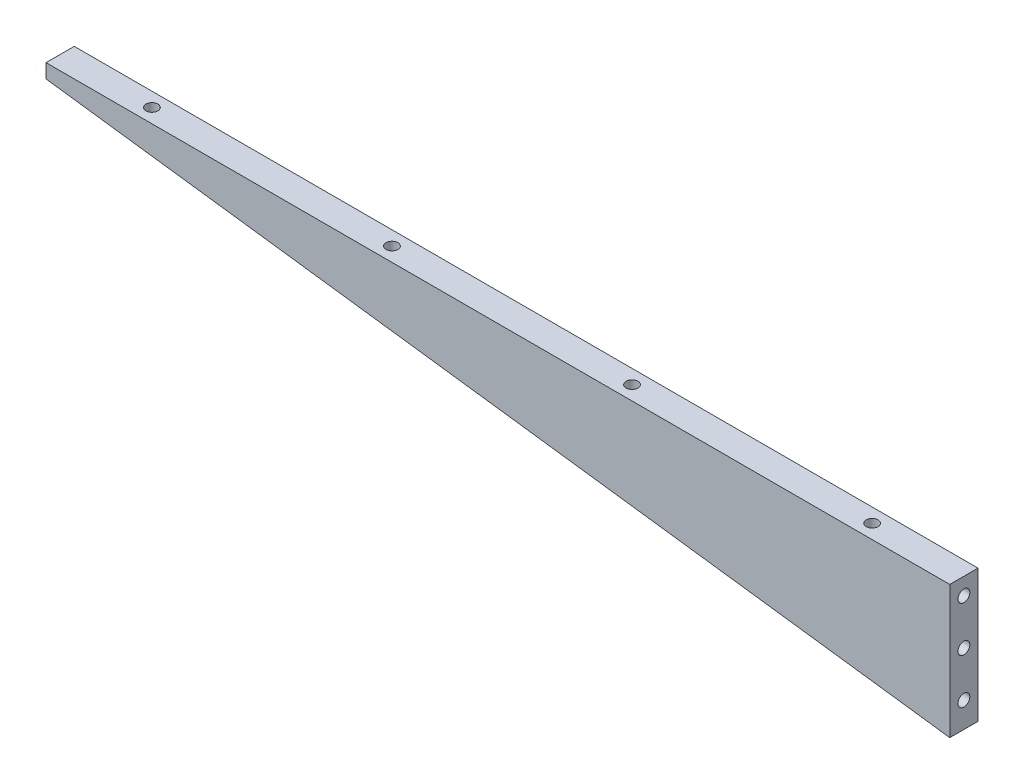
SolidWorks part; units mm, degrees
ref_plane "Front Plane" through (0, 0, 0) normal (0, 0, 1) x (1, 0, 0)
ref_plane "Top Plane" through (0, 0, 0) normal (0, 1, 0) x (1, 0, 0)
ref_plane "Right Plane" through (0, 0, 0) normal (1, 0, 0) x (0, 0, -1)
sketch "Sketch1" plane through (0, 0, 0) normal (0, 0, 1) x (1, 0, 0)
  line L0 (0, 0) -> (-320, 42)
  line L1 (-320, 47) -> (0, 47)
  line L2 (0, 47) -> (0, 0)
  line L3 (-320, 47) -> (-320, 42)
  dimension "D1" = 47
  dimension "D2" = 320
  dimension "D3" = 5
extrude "Boss-Extrude1" add sketch "Sketch1" along normal blind 10
hole_wizard "M5 Tapped Hole1" positions "Sketch3" profile "Sketch2" tap size "M5" standard "Gb"
sketch "Sketch3" plane through (0, 47, 0) normal (0, 1, 0) x (-1, 0, 0)
  line L0 (320, 10) -> (320, 0) construction
  line L1 (320, 5) -> (274.499, 5) construction
  point P0 (287.5, 5)
  point P19 (202.5, 5)
  point P20 (117.5, 5)
  point P21 (32.5, 5)
  dimension "D1" = 32.5
  dimension "D2" = 4
  dimension "D3" = 85
sketch "Sketch2" plane through (-287.5, 47, 5) normal (1, 0, 0) x (0, 0, 1)
  line L0 (0, 0) -> (0, 15.2618)
  line L1 (0, 15.2618) -> (2.1, 14)
  line L2 (2.1, 14) -> (2.1, 0)
  line L5 (2.1, 0) -> (0, 0)
  line L10 (0, 15.2618) -> (-2.1, 14) construction
  line L11 (0, -6.35) -> (0, 107.95) construction
  dimension "螺纹孔钻头直径" = 4.2
  dimension "螺纹孔钻头深度" = 14
  dimension "导头角度" = 118
cosmetic thread "Cosmetic Thread 1"
cosmetic thread "Cosmetic Thread 2"
cosmetic thread "Cosmetic Thread 3"
cosmetic thread "Cosmetic Thread 4"
hole_wizard "M5 Tapped Hole2" positions "Sketch5" profile "Sketch4" tap size "M5" standard "Gb"
sketch "Sketch5" plane through (0, 0, 0) normal (1, 0, 0) x (0, 0, -1)
  line L0 (-10, 47) -> (0, 47) construction
  line L1 (-5, 0) -> (-5, 55.6467) construction
  line L2 (-10, 0) -> (0, 0) construction
  point P0 (-5, 41)
  point P2 (-5, 25)
  point P4 (-5, 9)
  dimension "D1" = 6
  dimension "D2" = 16
  dimension "D3" = 16
sketch "Sketch4" plane through (0, 41, 5) normal (0, 1, 0) x (0, 0, -1)
  line L0 (0, 0) -> (0, 15.2618)
  line L1 (0, 15.2618) -> (2.1, 14)
  line L2 (2.1, 14) -> (2.1, 0)
  line L5 (2.1, 0) -> (0, 0)
  line L10 (0, 15.2618) -> (-2.1, 14) construction
  line L11 (0, -6.35) -> (0, 107.95) construction
  dimension "螺纹孔钻头直径" = 4.2
  dimension "螺纹孔钻头深度" = 14
  dimension "导头角度" = 118
cosmetic thread "Cosmetic Thread 5"
cosmetic thread "Cosmetic Thread 6"
cosmetic thread "Cosmetic Thread 7"
